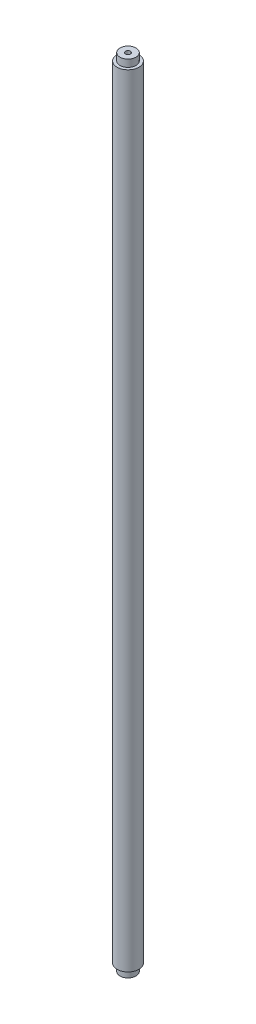
SolidWorks part; units mm, degrees
material "45"
ref_plane "Front Plane" through (0, 0, 0) normal (0, 0, 1) x (1, 0, 0)
ref_plane "Top Plane" through (0, 0, 0) normal (0, 1, 0) x (1, 0, 0)
ref_plane "Right Plane" through (0, 0, 0) normal (1, 0, 0) x (0, 0, -1)
sketch "Sketch1" plane through (0, 0, 0) normal (0, 1, 0) x (1, 0, 0)
  circle A0 centre (0, 0) radius 15
  dimension "D1" = 30
extrude "Boss-Extrude1" add sketch "Sketch1" along normal blind 1075
sketch "Sketch2" plane through (0, 1075, 0) normal (0, 1, 0) x (1, 0, 0)
  circle A0 centre (0, 0) radius 11
  dimension "D1" = 22
extrude "Boss-Extrude2" add sketch "Sketch2" along normal blind 10
sketch "Sketch3" plane through (0, 0, 0) normal (0, -1, 0) x (1, 0, 0)
  circle A0 centre (0, 0) radius 11
  dimension "D1" = 22
extrude "Boss-Extrude3" add sketch "Sketch3" along normal blind 10
hole_wizard "M8 Tapped Hole1" positions "Sketch4" profile "Sketch5" tap size "M8" standard "GB"
sketch "Sketch4" plane through (0, -10, 0) normal (0, -1, 0) x (-1, 0, 0)
  point P0 (0, 0)
cosmetic thread "Hole thread line1" parameters "D1"=16, "D2"=8
sketch "Sketch5" plane through (0, -10, 0) normal (1, 0, 0) x (0, 0, -1)
  line L0 (0, 0) -> (0, 21.7929)
  line L1 (0, 21.7929) -> (3.4, 19.75)
  line L2 (3.4, 19.75) -> (3.4, 0)
  line L5 (3.4, 0) -> (0, 0)
  line L10 (0, 21.7929) -> (-3.4, 19.75) construction
  line L11 (0, -6.35) -> (0, 107.95) construction
  dimension "螺纹孔钻头直径" = 6.8
  dimension "螺纹孔钻头深度" = 19.75
  dimension "导头角度" = 118
hole_wizard "M8 Tapped Hole2" positions "Sketch6" profile "Sketch7" tap size "M8" standard "GB"
sketch "Sketch6" plane through (0, 1085, 0) normal (0, 1, 0) x (1, 0, 0)
  point P0 (0, 0)
sketch "Sketch7" plane through (0, 1085, 0) normal (1, 0, 0) x (0, 0, 1)
  line L0 (0, 0) -> (0, 21.7929)
  line L1 (0, 21.7929) -> (3.4, 19.75)
  line L2 (3.4, 19.75) -> (3.4, 0)
  line L5 (3.4, 0) -> (0, 0)
  line L10 (0, 21.7929) -> (-3.4, 19.75) construction
  line L11 (0, -6.35) -> (0, 107.95) construction
  dimension "螺纹孔钻头直径" = 6.8
  dimension "螺纹孔钻头深度" = 19.75
  dimension "导头角度" = 118
cosmetic thread "Hole thread line2" parameters "D1"=16, "D2"=8
